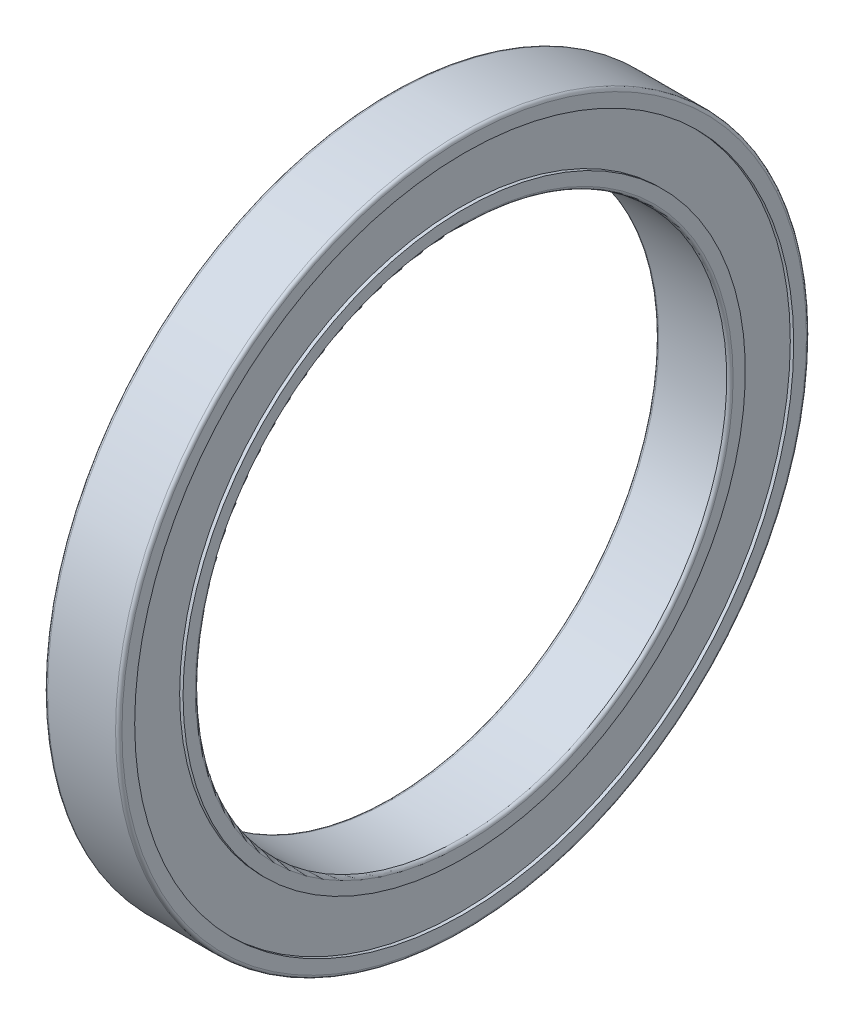
from build123d import *

# Parameters (mm, degrees)
FILLET1_R = 0.3
FILLET2_R = 0.3


with BuildPart() as part:
    # Sketch1 → Revolve1 (revolve)
    with BuildSketch(Plane.XY, mode=Mode.PRIVATE) as revolve1_sk:
        Polygon((0, 25), (7, 25), (7, 26.45), (6.68, 26.45), (6.68, 31), (7, 31), (7, 32.5), (0, 32.5), (0, 31), (0.32, 31), (0.32, 26.45), (0, 26.45), align=None)
    revolve(revolve1_sk.sketch.rotate(Axis((0, 0, 0), (1, 0, 0)), 90), axis=Axis((0, 0, 0), (1, 0, 0)))

    # Fillet1
    fillet1_edges = [part.edges().sort_by_distance(p)[0] for p in [
        (0, 0, -32.5),
        (7, 0, -32.5),
    ]]
    fillet(fillet1_edges, radius=FILLET1_R)

    # Fillet2
    fillet2_edges = [part.edges().sort_by_distance(p)[0] for p in [
        (7, 0, -25),
        (0, 0, -25),
    ]]
    fillet(fillet2_edges, radius=FILLET2_R)


solid = part.part
